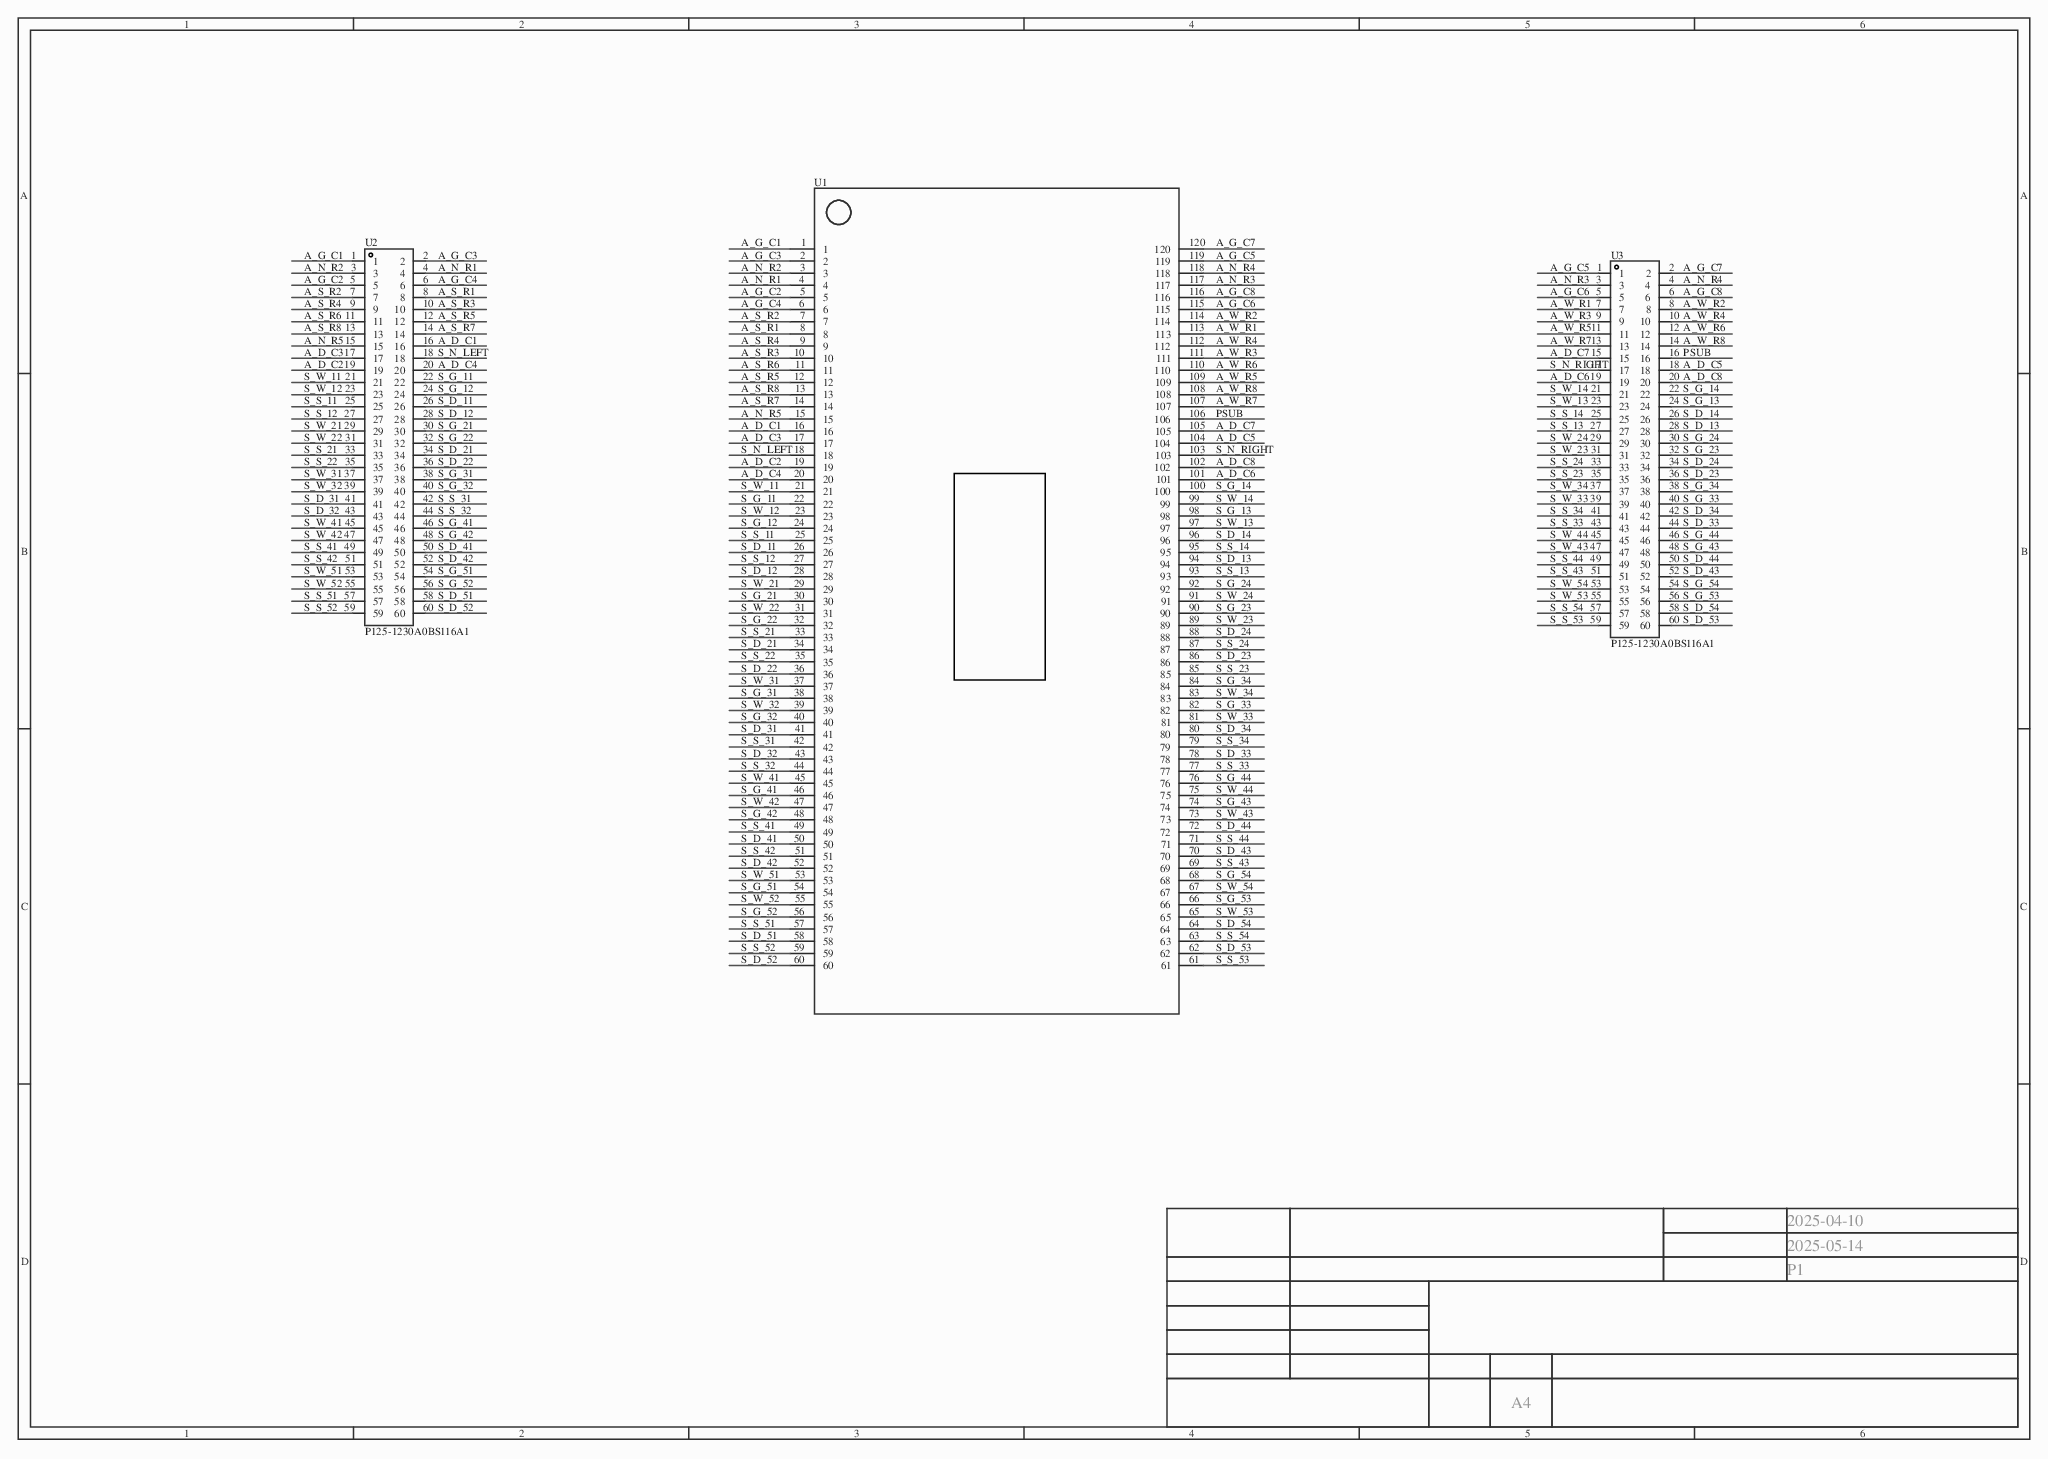
[diagram p0: MISC82787-2.schdoc]
# Altium project MISC82787-7.PrjPCB
1 sheet, 3 parts. Net scope: global (net labels, ports and power ports of the same name join across sheets).
Board file: MISC82787.pcbdoc

## Sheet MISC82787-2.schdoc
size 429 x 307 mm; Version: V1.0; @Project Name: MISC82787; @Page Count: 1; @Update Date: 2025-05-14; @Create Date: 2025-04-10; @Schematic Name: MISC82787; @Page No: 1; @Create Time: 08:49:59; @Update Time: 15:03:46

### Parts
U1  (no value)  [XP]
U2  P125-1230A0BS116A1  [HDR-TH_60P-P2.54-V-M-R2-C30-S2.54-1]
U3  P125-1230A0BS116A1  [HDR-TH_60P-P2.54-V-M-R2-C30-S2.54-1]

### Nets
A_D_C1: U1.16 U2.16
A_D_C2: U1.19 U2.19
A_D_C3: U1.17 U2.17
A_D_C4: U1.20 U2.20
A_D_C5: U1.104 U3.18
A_D_C6: U1.101 U3.19
A_D_C7: U1.105 U3.15
A_D_C8: U1.102 U3.20
A_G_C1: U1.1 U2.1
A_G_C2: U1.5 U2.5
A_G_C3: U1.2 U2.2
A_G_C4: U1.6 U2.6
A_G_C5: U1.119 U3.1
A_G_C6: U1.115 U3.5
A_G_C7: U1.120 U3.2
A_G_C8: U1.116 U3.6
A_N_R1: U1.4 U2.4
A_N_R2: U1.3 U2.3
A_N_R3: U1.117 U3.3
A_N_R4: U1.118 U3.4
A_N_R5: U1.15 U2.15
A_S_R1: U1.8 U2.8
A_S_R2: U1.7 U2.7
A_S_R3: U1.10 U2.10
A_S_R4: U1.9 U2.9
A_S_R5: U1.12 U2.12
A_S_R6: U1.11 U2.11
A_S_R7: U1.14 U2.14
A_S_R8: U1.13 U2.13
A_W_R1: U1.113 U3.7
A_W_R2: U1.114 U3.8
A_W_R3: U1.111 U3.9
A_W_R4: U1.112 U3.10
A_W_R5: U1.109 U3.11
A_W_R6: U1.110 U3.12
A_W_R7: U1.107 U3.13
A_W_R8: U1.108 U3.14
PSUB: U1.106 U3.16
S_D_11: U1.26 U2.26
S_D_12: U1.28 U2.28
S_D_13: U1.94 U3.28
S_D_14: U1.96 U3.26
S_D_21: U1.34 U2.34
S_D_22: U1.36 U2.36
S_D_23: U1.86 U3.36
S_D_24: U1.88 U3.34
S_D_31: U1.41 U2.41
S_D_32: U1.43 U2.43
S_D_33: U1.78 U3.44
S_D_34: U1.80 U3.42
S_D_41: U1.50 U2.50
S_D_42: U1.52 U2.52
S_D_43: U1.70 U3.52
S_D_44: U1.72 U3.50
S_D_51: U1.58 U2.58
S_D_52: U1.60 U2.60
S_D_53: U1.62 U3.60
S_D_54: U1.64 U3.58
S_G_11: U1.22 U2.22
S_G_12: U1.24 U2.24
S_G_13: U1.98 U3.24
S_G_14: U1.100 U3.22
S_G_21: U1.30 U2.30
S_G_22: U1.32 U2.32
S_G_23: U1.90 U3.32
S_G_24: U1.92 U3.30
S_G_31: U1.38 U2.38
S_G_32: U1.40 U2.40
S_G_33: U1.82 U3.40
S_G_34: U1.84 U3.38
S_G_41: U1.46 U2.46
S_G_42: U1.48 U2.48
S_G_43: U1.74 U3.48
S_G_44: U1.76 U3.46
S_G_51: U1.54 U2.54
S_G_52: U1.56 U2.56
S_G_53: U1.66 U3.56
S_G_54: U1.68 U3.54
S_N_LEFT: U1.18 U2.18
S_N_RIGHT: U1.103 U3.17
S_S_11: U1.25 U2.25
S_S_12: U1.27 U2.27
S_S_13: U1.93 U3.27
S_S_14: U1.95 U3.25
S_S_21: U1.33 U2.33
S_S_22: U1.35 U2.35
S_S_23: U1.85 U3.35
S_S_24: U1.87 U3.33
S_S_31: U1.42 U2.42
S_S_32: U1.44 U2.44
S_S_33: U1.77 U3.43
S_S_34: U1.79 U3.41
S_S_41: U1.49 U2.49
S_S_42: U1.51 U2.51
S_S_43: U1.69 U3.51
S_S_44: U1.71 U3.49
S_S_51: U1.57 U2.57
S_S_52: U1.59 U2.59
S_S_53: U1.61 U3.59
S_S_54: U1.63 U3.57
S_W_11: U1.21 U2.21
S_W_12: U1.23 U2.23
S_W_13: U1.97 U3.23
S_W_14: U1.99 U3.21
S_W_21: U1.29 U2.29
S_W_22: U1.31 U2.31
S_W_23: U1.89 U3.31
S_W_24: U1.91 U3.29
S_W_31: U1.37 U2.37
S_W_32: U1.39 U2.39
S_W_33: U1.81 U3.39
S_W_34: U1.83 U3.37
S_W_41: U1.45 U2.45
S_W_42: U1.47 U2.47
S_W_43: U1.73 U3.47
S_W_44: U1.75 U3.45
S_W_51: U1.53 U2.53
S_W_52: U1.55 U2.55
S_W_53: U1.65 U3.55
S_W_54: U1.67 U3.53

### Notes on the sheet
- 1
- 2
- 3
- 4
- 5
- 6
- A
- B
- C
- 2025-04-10
- 2025-05-14
- D
- P1
- A4

### Library data of the parts
U1 = Chip3Array: Add into BOM: yes; Symbol: Chip3Array; Device: Chip3Array; Convert to PCB: yes
U2 U3 = P125-1230A0BS116A1: Add into BOM: yes; Pin Structure: 2x30P; Pitch: 2.54mm; Symbol: P125-1230A0BS116A1; Device: P125-1230A0BS116A1; Supplier Part: C19190515; Manufacturer Part: P125-1230A0BS116A1; Datasheet: https://atta.szlcsc.com/upload/public/pdf/source/20231110/933F8D648B10E9101EFC894132A28518.pdf; Supplier: LCSC; Convert to PCB: yes; Row Spacing: 2.54mm; Number of Pins: 60P; Length of Mating Pin: 6mm; Insulation Height: 2.5mm; Length of End Connection Pin: 3mm